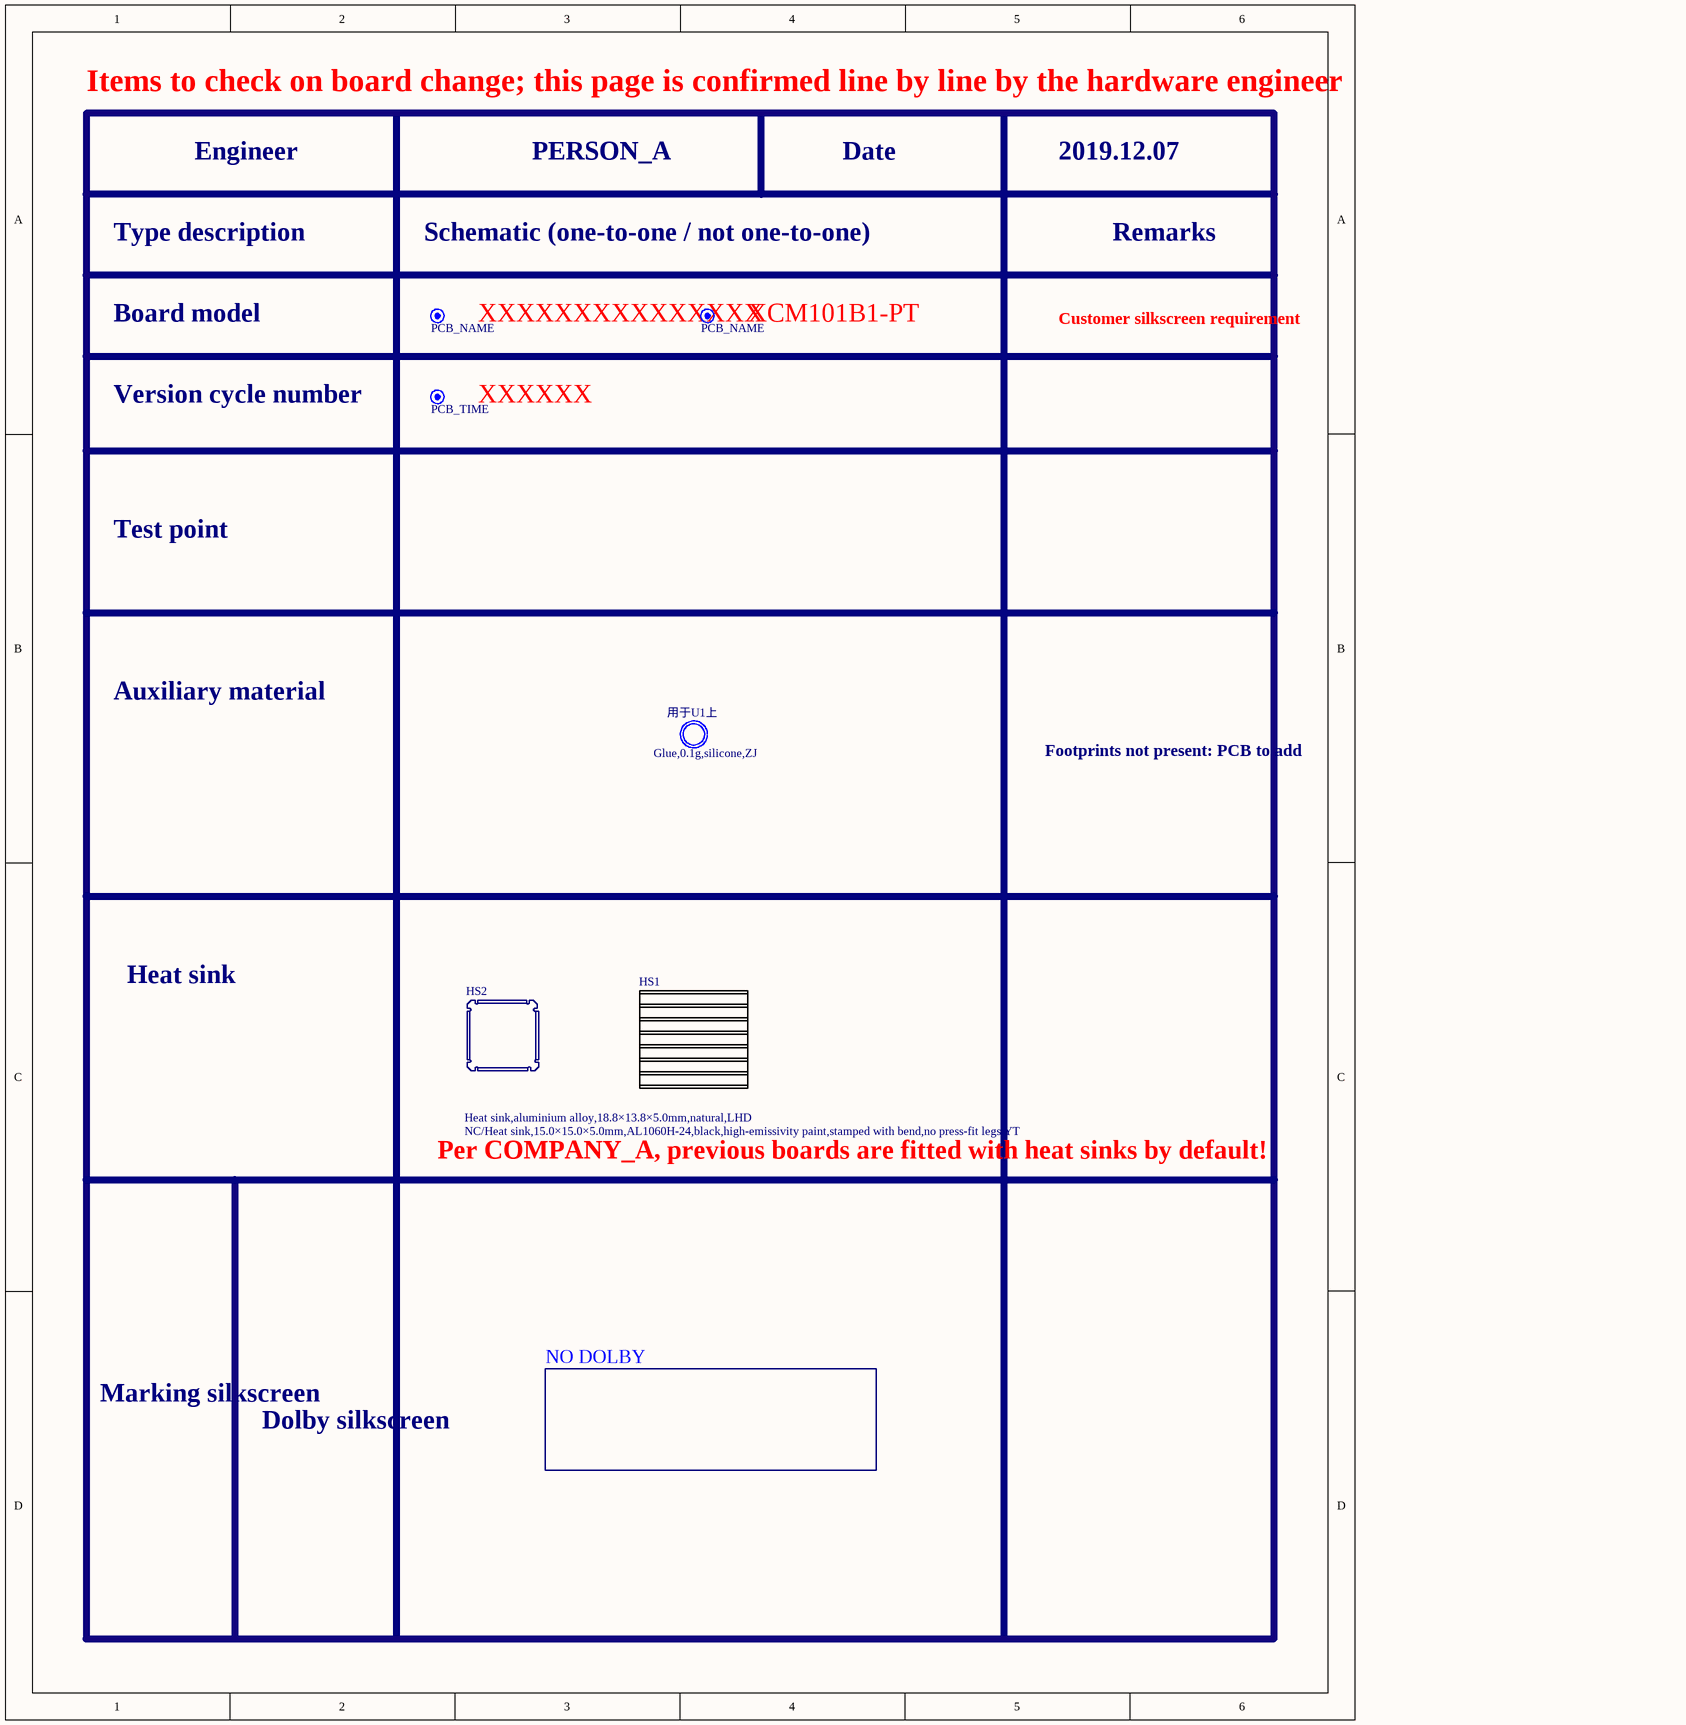
[diagram p0: MISC86383-6.SchDoc]
# Altium schematic sheet MISC86383-6.SchDoc
size 254 x 322 mm

## Parts
HS1  Heat sink,aluminium alloy,18.8×13.8×5.0mm,natural,LHD  [HS(18.8*13.8*5)]
HS2  NC/Heat sink,15.0×15.0×5.0mm,AL1060H-24,black,high-emissivity paint,stamped with bend,no press-fit legs,YT  [HS(15X15X5)-S]
NO_DOLBY  NO DOLBY  [NO DOLBY-SILK]
XCM101B1-PT  PCB_NAME  [PCB_NAME]
XXXXXX  PCB_TIME  [PCB_TIME]
XXXXXXXXXXXXXXX  PCB_NAME  [PCB_NAME]
用于U1上  Glue,0.1g,silicone,ZJ  [Heat-Shrinkable Tube]

## Notes on the sheet
- Items to check on board change; this page is confirmed line by line by the hardware engineer
- Engineer
- PERSON_A
- Date
- 2019.12.07
- Type description
- Schematic (one-to-one / not one-to-one)
- Remarks
- Board model
- Customer silkscreen requirement
- Version cycle number
- Test point
- Auxiliary material
- Footprints not present: PCB to add
- Heat sink
- Per COMPANY_A, previous boards are fitted with heat sinks by default!
- Marking silkscreen
- Dolby silkscreen

## Library data of the parts
HS1 = 18.8×13.8×5-本色-THD-HS: SMD heat sink
HS2 = 004.040.0008928-D: Heat sink,15.0×15.0×5.0mm,AL1060H-24,black,high-emissivity paint,stamped with bend,no press-fit legs,YT-D
用于U1上 = Φ12mm×12mm-黑色-125度(UL认证)-D